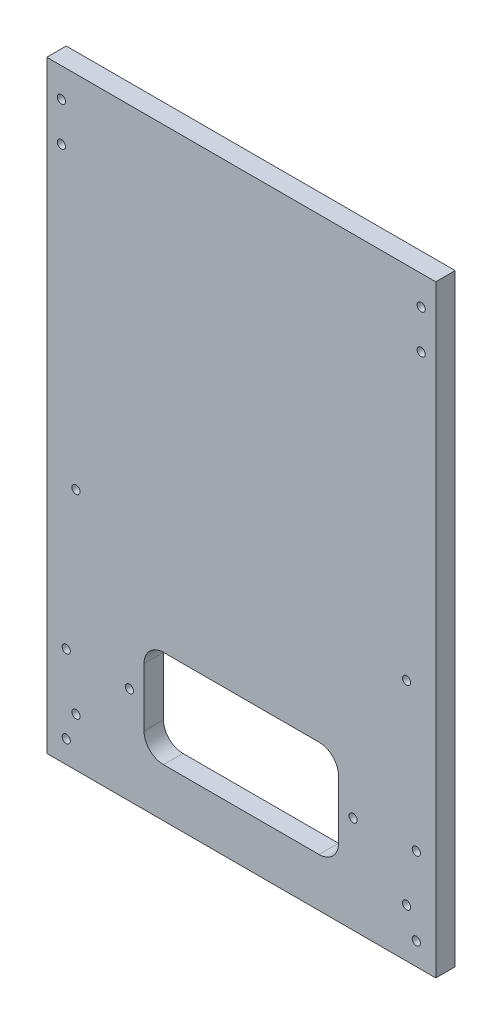
SolidWorks part; units mm, degrees
material "黄茶色亚克力"
ref_plane "前视基准面" through (0, 0, 0) normal (0, 0, 1) x (1, 0, 0)
ref_plane "上视基准面" through (0, 0, 0) normal (0, 1, 0) x (1, 0, 0)
ref_plane "右视基准面" through (0, 0, 0) normal (1, 0, 0) x (0, 0, -1)
sketch "草图1" plane through (0, 0, 0) normal (0, 0, 1) x (1, 0, 0)
  line L1 (-100, -155) -> (100, -155)
  line L2 (-100, -155) -> (-100, 155)
  line L3 (-100, 155) -> (100, 155)
  line L4 (100, -155) -> (100, 155)
  line L5 (-100, -155) -> (100, 155) construction
  line L6 (-100, 155) -> (100, -155) construction
  point P0 (0, 0)
  dimension "D1" = 200
  dimension "D2" = 310
extrude "凸台-拉伸1" add sketch "草图1" along normal mid plane 10
sketch "草图2" plane through (0, 0, 5) normal (0, 0, 1) x (1, 0, 0)
  line L0 (0, 155) -> (0, -250.1977) construction
  line L1 (50, -130) -> (-50, -130)
  line L2 (50, -130) -> (50, -80)
  line L3 (50, -80) -> (-50, -80)
  line L4 (-50, -130) -> (-50, -80)
  line L5 (100, 155) -> (-100, 155) construction
  line L6 (-100, -155) -> (100, -155) construction
  dimension "D1" = 100
  dimension "D2" = 50
  dimension "D3" = 25
extrude "切除-拉伸1" cut sketch "草图2" against normal through all
hole_wizard "M5 螺纹孔2" positions "草图7" profile "草图8" tap size "M5" standard "ISO" end condition through all
sketch "草图7" plane through (0, 0, 5) normal (0, 0, 1) x (1, 0, 0)
  point P0 (85, -130)
  point P3 (85, -30)
  point P6 (-85, -30)
  point P9 (-85, -130)
sketch "草图8" plane through (85, -130, 5) normal (1, 0, 0) x (0, -1, 0)
  line L0 (0, 0) -> (0, 10)
  line L1 (0, 10) -> (2.1, 10)
  line L2 (2.1, 10) -> (2.1, 0)
  line L5 (2.1, 0) -> (0, 0)
  line L11 (0, -6.35) -> (0, 107.95) construction
  dimension "通孔螺纹孔钻头直径" = 4.2
  dimension "通孔螺纹孔钻头深度" = 10
cosmetic thread "孔螺蚊线8" parameters "D2"=5
cosmetic thread "孔螺蚊线9" parameters "D2"=5
cosmetic thread "孔螺蚊线10" parameters "D2"=5
cosmetic thread "孔螺蚊线11" parameters "D2"=5
fillet "圆角1" radius 10 4 edges at (50, -80, 0) (-50, -80, 0) (-50, -130, 0) (50, -130, 0)
hole_wizard "M5 螺纹孔4" positions "草图14" profile "草图15" tap size "M5" standard "GB" end condition up to next
sketch "草图14" plane through (0, 0, -5) normal (0, 0, -1) x (-1, 0, 0)
  point P0 (92.5, 120)
  point P3 (92.5, 140)
  point P6 (-92.5, 140)
  point P9 (-92.5, 120)
sketch "草图15" plane through (-92.5, 120, -5) normal (1, 0, 0) x (0, 1, 0)
  line L0 (0, 0) -> (0, 10)
  line L1 (0, 10) -> (2.1, 10)
  line L2 (2.1, 10) -> (2.1, 0)
  line L5 (2.1, 0) -> (0, 0)
  line L11 (0, -6.35) -> (0, 107.95) construction
  dimension "通孔螺纹孔钻头直径" = 4.2
  dimension "通孔螺纹孔钻头深度" = 10
cosmetic thread "孔螺蚊线18" parameters "D2"=5
cosmetic thread "孔螺蚊线19" parameters "D2"=5
cosmetic thread "孔螺蚊线20" parameters "D2"=5
cosmetic thread "孔螺蚊线21" parameters "D2"=5
hole_wizard "M5 螺纹孔5" positions "草图16" profile "草图17" tap size "M5" standard "ISO" end condition through all
sketch "草图16" plane through (0, 0, -5) normal (0, 0, -1) x (-1, 0, 0)
  line L0 (57.5, -118.25) -> (57.5, -91.75) construction
  line L2 (-57.5, -118.25) -> (-57.5, -91.75) construction
  arc A0 (54.25, -115) -> (60.75, -115) centre (57.5, -115) ccw construction
  arc A1 (60.75, -95) -> (54.25, -95) centre (57.5, -95) ccw construction
  arc A2 (-60.75, -115) -> (-54.25, -115) centre (-57.5, -115) ccw construction
  arc A3 (-54.25, -95) -> (-60.75, -95) centre (-57.5, -95) ccw construction
  point P2 (-57.5, -105)
  point P34 (57.5, -105)
sketch "草图17" plane through (57.5, -105, -5) normal (1, 0, 0) x (0, 1, 0)
  line L0 (0, 0) -> (0, 10)
  line L1 (0, 10) -> (2.1, 10)
  line L2 (2.1, 10) -> (2.1, 0)
  line L5 (2.1, 0) -> (0, 0)
  line L11 (0, -6.35) -> (0, 107.95) construction
  dimension "通孔螺纹孔钻头直径" = 4.2
  dimension "通孔螺纹孔钻头深度" = 10
cosmetic thread "孔螺蚊线22" parameters "D2"=5
cosmetic thread "孔螺蚊线23" parameters "D2"=5
hole_wizard "M5 螺纹孔6" positions "草图18" profile "草图19" tap size "M5" standard "GB" end condition through all
sketch "草图18" plane through (0, 0, -5) normal (0, 0, -1) x (-1, 0, 0)
  point P0 (90, -143.5)
  point P3 (90, -103.5)
  point P6 (-90, -103.5)
  point P9 (-90, -143.5)
sketch "草图19" plane through (-90, -143.5, -5) normal (1, 0, 0) x (0, 1, 0)
  line L0 (0, 0) -> (0, 10)
  line L1 (0, 10) -> (2.1, 10)
  line L2 (2.1, 10) -> (2.1, 0)
  line L5 (2.1, 0) -> (0, 0)
  line L11 (0, -6.35) -> (0, 107.95) construction
  dimension "通孔螺纹孔钻头直径" = 4.2
  dimension "通孔螺纹孔钻头深度" = 10
cosmetic thread "孔螺蚊线24" parameters "D2"=5
cosmetic thread "孔螺蚊线25" parameters "D2"=5
cosmetic thread "孔螺蚊线26" parameters "D2"=5
cosmetic thread "孔螺蚊线27" parameters "D2"=5
